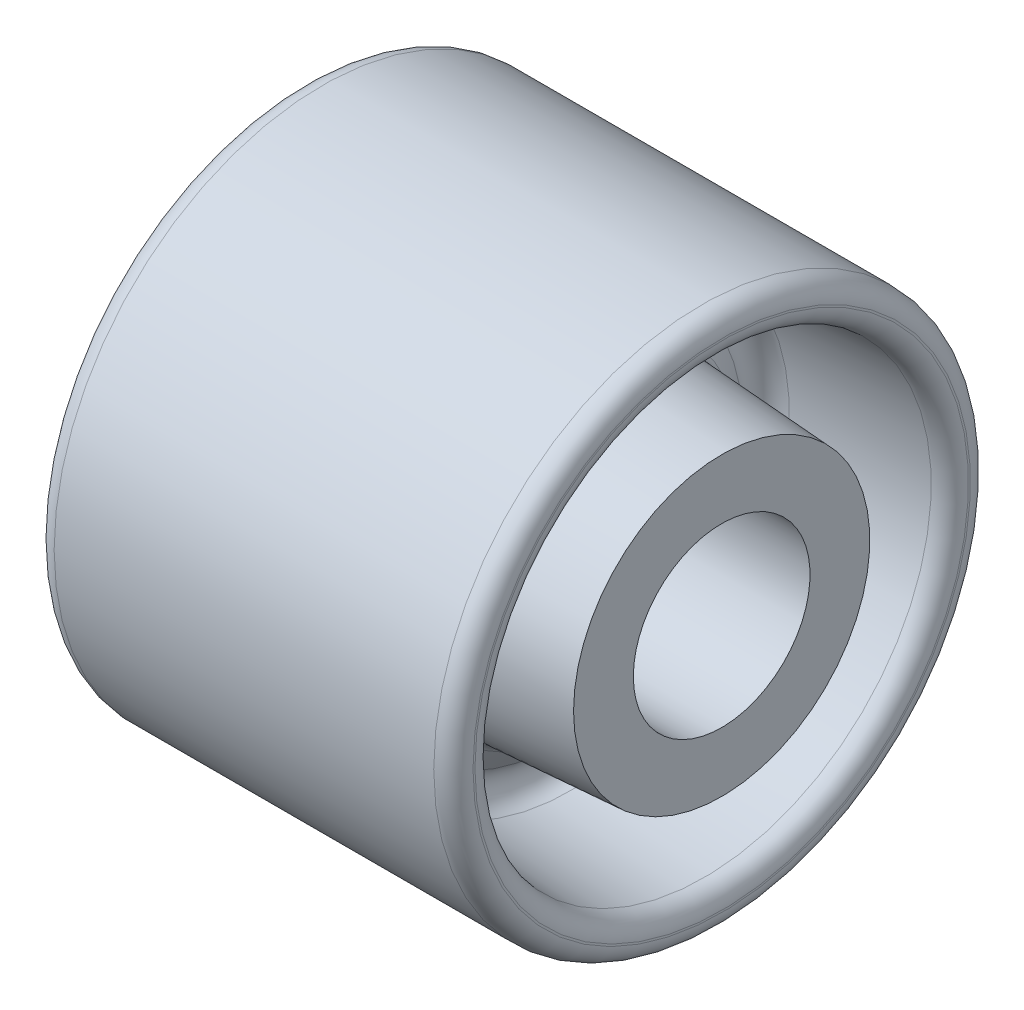
SolidWorks part; units mm, degrees
ref_plane "Front Plane" through (0, 0, 0) normal (0, 0, 1) x (1, 0, 0)
ref_plane "Top Plane" through (0, 0, 0) normal (0, 1, 0) x (1, 0, 0)
ref_plane "Right Plane" through (0, 0, 0) normal (1, 0, 0) x (0, 0, -1)
sketch "Sketch1" plane through (0, 0, 0) normal (0, 1, 0) x (1, 0, 0)
  line L0 (-35.4182, 0) -> (28.5818, 0)
  line L1 (-35.4182, 3) -> (-35.4182, 5.8153)
  line L2 (28.5818, 3) -> (28.5818, 5.8153)
  line L3 (-35.4182, 5.8153) -> (-35.4182, 8.5)
  line L4 (-35.4182, 24.5) -> (-35.4182, 24.2055)
  line L5 (-39.4295, -13.5) -> (38.2665, -13.5) construction
  line L6 (25.5818, 27.5) -> (-32.4182, 27.5)
  line L7 (28.5818, 24.2055) -> (28.5818, 24.5)
  line L8 (-10.1342, 18.8549) -> (-7.1342, 15.3323)
  line L9 (3.2979, 14.9646) -> (6.2979, 11.442)
  line L10 (-35.4182, 3) -> (-35.4182, 0)
  line L11 (28.5818, 5.8153) -> (28.5818, 9.1343)
  line L12 (28.5818, 3) -> (28.5818, 0)
  arc A0 (-35.4182, 8.5) -> (-9.3303, 10.3885) centre (-0.4182, -293.8622) cw
  arc A1 (25.8771, 21.22) -> (5.4921, 19.9084) centre (-3.4182, 317.4461) cw
  arc A2 (-12.3284, 19.9084) -> (-32.7134, 21.22) centre (-3.4182, 317.4461) cw
  arc A3 (8.494, 10.3885) -> (28.5818, 9.1343) centre (-0.4182, -293.8622) cw
  arc A4 (-10.1342, 18.8549) -> (-12.3284, 19.9084) centre (-12.4182, 16.9097) ccw
  arc A5 (3.2979, 14.9646) -> (5.4921, 19.9084) centre (5.5818, 16.9097) cw
  arc A6 (6.2979, 11.442) -> (8.494, 10.3885) centre (8.5818, 13.3872) ccw
  arc A7 (-7.1342, 15.3323) -> (-9.3303, 10.3885) centre (-9.4182, 13.3872) cw
  arc A8 (-35.4182, 24.2055) -> (-32.7134, 21.22) centre (-32.4182, 24.2055) ccw
  arc A11 (-35.4182, 24.5) -> (-32.4182, 27.5) centre (-32.4182, 24.5) cw
  arc A12 (28.5818, 24.5) -> (25.5818, 27.5) centre (25.5818, 24.5) ccw
  arc A13 (25.8771, 21.22) -> (28.5818, 24.2055) centre (25.5818, 24.2055) ccw
  point P8 (-11.0001, 19.8716)
  point P22 (7.1645, 10.4245)
  point P27 (-35.4182, 21.5)
  point P30 (-35.4182, 8.5)
  point P33 (-35.4182, 0)
  point P36 (-35.4182, 27.5)
  point P39 (28.5818, 27.5)
  point P42 (28.5818, 21.5)
  point P45 (28.5818, 9.1343)
  point P48 (28.5818, 0.6343)
  dimension "D1" = 8.5
  dimension "D2" = 8.5
  dimension "D3" = 19
  dimension "D4" = 6
  dimension "D5" = 6
  dimension "D6" = 3
  dimension "D7" = 64
  dimension "D8" = 58
revolve "Revolve1" add sketch "Sketch1" angle 360 about L5
